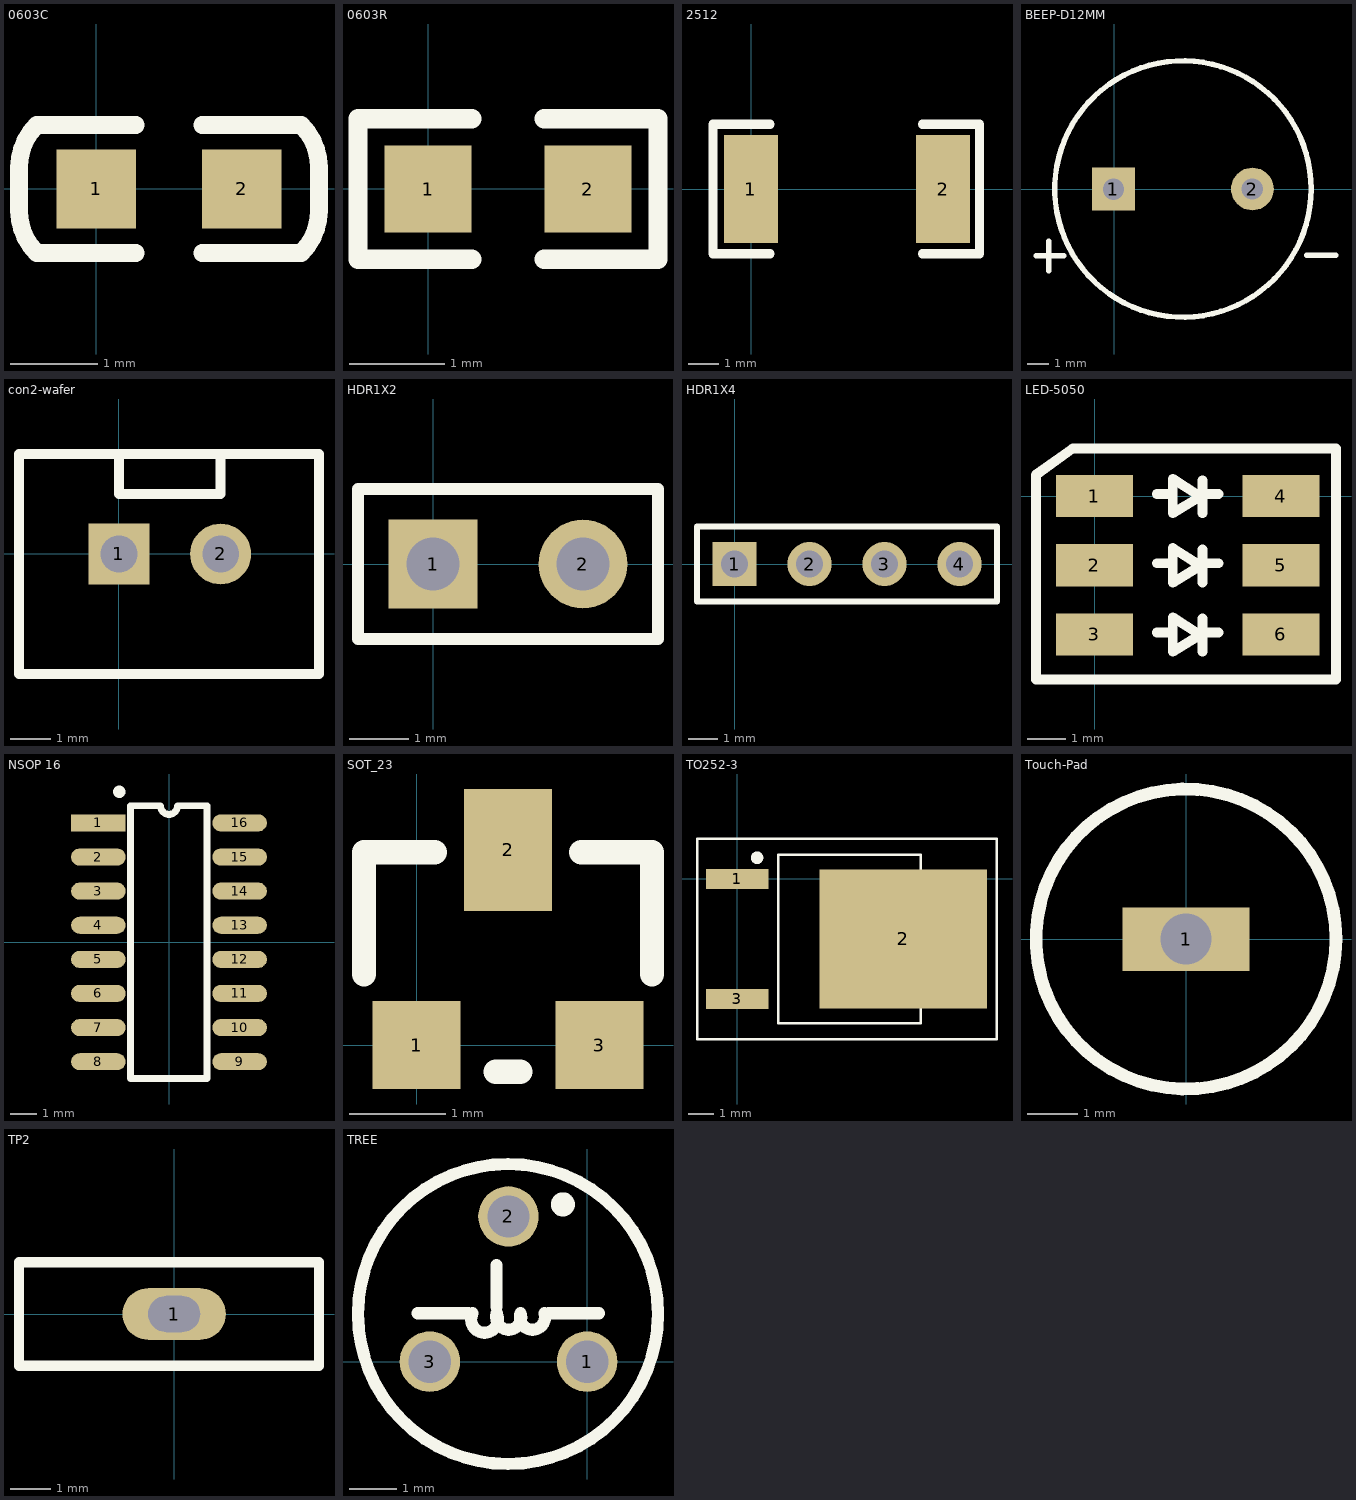
[diagram p0: the footprints below, top view; thin cyan lines are the x and y axes]
# Altium footprint library MISC75988-2.PcbLib: 14 footprints
Each footprint in its own frame and in the unit in brackets; x right, y up, seen from the top. Pads: shape width x height; smd on the part's side, far side on the other; paste and mask are expansions set on the pad; w line width, h text height; cw(c..) or ccw(c..) is an arc to the next point about the centre after c.

## 0603C [mil]
height 62.99
pads (2):
  rect 36x36 smd: 1(0,0) 2(66,0)
Top Overlay:
  lines w8: 18,-29 -27,-29 cw(c-7.69,-9.69) -35,-9.69 -35,9.69 cw(c-7.69,9.69) -27,29 18,29 ; 48,-29 93,-29 ccw(c73.69,-9.69) 101,-9.69 101,9.69 ccw(c73.69,9.69) 93,29 48,29

## 0603R [mil]
height 62.99
pads (2):
  rect 36x36 smd: 1(0,0) 2(66,0)
Top Overlay:
  lines w8: 18,-29 -29,-29 -29,29 18,29 ; 48,-29 95,-29 95,29 48,29

## 2512 [mm]
height 1.6
pads (2):
  rect 1.8x3.6 smd: 1(0,0) 2(6.4,0)
Top Overlay:
  lines w0.305: 0.635,-2.159 -1.27,-2.159 -1.27,2.159 0.635,2.159 ; 5.715,-2.159 7.62,-2.159 7.62,2.159 5.715,2.159

## BEEP-D12MM [mm]
pads (2):
  rect 2x2 hole 1: 1(-0.026,-0.004)
  round 2 hole 1: 2(6.477,0)
Top Overlay:
  circle w0.254: c3.227,0 r6
  lines w0.254: -3.653,-3.134 -2.353,-3.134 ; -3.053,-3.834 -3.053,-2.434 ; 9.029,-3.11 10.389,-3.11

## con2-wafer [mil]
height 62.99
pads (2):
  rect 60x60 hole 36: 1(0,0)
  round 60 hole 36: 2(100,0)
Top Overlay:
  lines w10: -98.42,-9.84 -98.42,98.42 196.85,98.42 196.85,-118.11 -98.42,-118.11 -98.42,0 ; 0,98.42 0,59.05 100,59.05 100,98.03

## HDR1X2 [mm] "Connector; Header; 2 Position"
pads (2):
  rect 1.5x1.5 hole 0.9: 1(0,0)
  round 1.5 hole 0.9: 2(2.54,0)
Top Overlay:
  lines w0.2: -1.27,-1.27 -1.27,1.27 3.81,1.27 3.81,-1.27 -1.27,-1.27

## HDR1X4 [mm] "Connector; Header; 4 Position"
pads (4):
  rect 1.5x1.5 hole 0.9: 1(0,0)
  round 1.5 hole 0.9: 2(2.54,0) 3(5.08,0) 4(7.62,0)
Top Overlay:
  lines w0.2: -1.27,-1.27 8.89,-1.27 8.89,1.27 -1.27,1.27 -1.27,-1.27

## LED-5050 [mm]
pads (6):
  rect 2x1.1 smd: 1(-0.004,0.009) 2(-0.004,-1.791) 3(-0.004,-3.591) 4(4.846,0.009) 5(4.846,-1.791) 6(4.846,-3.591)
Top Overlay:
  lines w0.254: 1.621,-3.541 2.021,-3.541 ; 1.621,-1.741 2.021,-1.741 ; 1.621,0.059 2.021,0.059 ; 2.709,-3.629 2.034,-4.041 2.034,-3.141 2.709,-3.579 ; 2.709,-1.829 2.034,-2.241 2.034,-1.341 2.709,-1.779 ; 2.709,-0.029 2.034,-0.441 2.034,0.459 2.709,0.021 ; 2.809,-4.041 2.809,-3.179 ; 2.809,-2.241 2.809,-1.379 ; 2.809,-0.441 2.809,0.421 ; 2.821,-3.541 3.221,-3.541 ; 2.821,-1.741 3.221,-1.741 ; 2.821,0.059 3.221,0.059 ; -1.521,-4.759 -1.521,0.562 -0.564,1.241 6.279,1.241 6.279,-4.759 -1.521,-4.759

## NSOP 16 [mil]
height 68.9
pads (16):
  rect 80x25 smd: 1(-103.5,175)
  oval 80x25 smd: 2(-103.5,125) 3(-103.5,75) 4(-103.5,25) 5(-103.5,-25) 6(-103.5,-75) 7(-103.5,-125) 8(-103.5,-175) 9(103.5,-175) 10(103.5,-125) 11(103.5,-75) 12(103.5,-25) 13(103.5,25) 14(103.5,75) 15(103.5,125) 16(103.5,175)
Top Overlay:
  circle w10: c-72.96,220.65 r4.07
  lines w10: -56.47,-199.52 -56.47,200.06 -12.5,200 ccw(c0,200) 12.5,200 55.47,200.06 55.47,-199.51 -56.47,-199.52

## SOT_23 [mil]
pads (3):
  rect 36x36 smd: 1(0,0) 3(75,0)
  rect 36x50 smd: 2(37.5,80)
Top Overlay:
  lines w10: -21.55,29 -21.55,79 7.5,79 ; 32.5,-11 42.5,-11 ; 67.5,79 96.56,79 96.56,29

## TO252-3 [mm] "D-PAK, 3-Pads, Body 5.7x6.7mm (max),"
height 2.39
pads (3):
  rect 2.5x0.8 smd: 1(0,0) 3(0,-4.8)
  rect 6.7x5.55 smd: 2(6.65,-2.4)
Top Overlay:
  circle w0.25: c0.8,0.85 r0.125
  lines w0.1: -1.6,-6.4 10.4,-6.4 10.4,1.6 -1.6,1.6 -1.6,-6.4 ; 1.65,-5.775 7.34,-5.775 7.34,0.975 1.65,0.975 1.65,-5.775

## Touch-Pad [mil]
height 62.99
pads (1):
  rect 100x50 hole 40: 1(0,0)
Top Overlay:
  circle w10: c0,0 r118.11

## TP2 [mil]
pads (1):
  oval 100x50 hole 35 slot 50 at 0 deg: 1(0,0)
Top Overlay:
  lines w10: -150,-50 -150,50 140,50 140,-50 -150,-50

## TREE [mil]
height 80
pads (3):
  round 50 hole 35: 1(0,0) 2(-65,120) 3(-130,0)
Top Overlay:
  circle w10: c-20,130 r5
  circle w10: c-65.39,39.37 r124.02
  lines w10: -140,40 -98.19,40 ; -94.68,40.02 ccw(c-84.85,34.95) -75,40 ; -75,45 -75,80 ; -74.68,40.02 ccw(c-64.84,36.73) -55,40 ccw(c-45.16,36.71) -35.32,39.98 ; -31.81,40 10,40